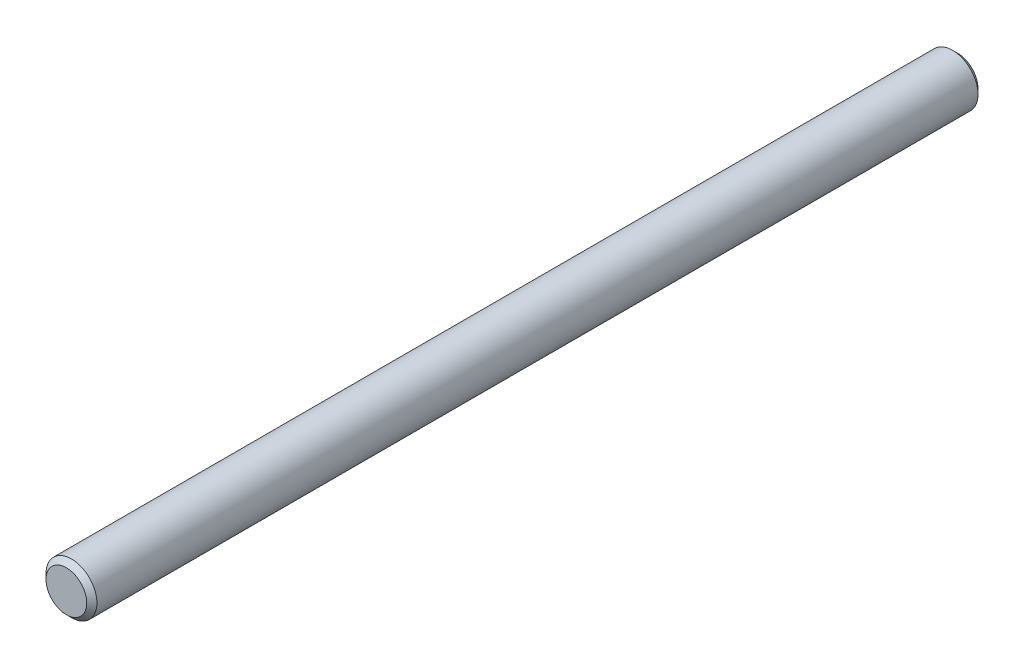
from build123d import *

# Parameters (mm, degrees)
SKETCH1_R           = 1
BOSS_EXTRUDE1_DEPTH = 17.5
CHAMFER1_SIZE       = 0.2


with BuildPart() as part:
    # Sketch1 → Boss-Extrude1 (new, symmetric)
    with BuildSketch(Plane.XY):
        Circle(SKETCH1_R)
    extrude(amount=BOSS_EXTRUDE1_DEPTH, both=True)

    # Chamfer1
    chamfer1_edges = [part.edges().sort_by_distance(p)[0] for p in [
        (-1, 0, -17.5),
        (-1, 0, 17.5),
    ]]
    chamfer(chamfer1_edges, length=CHAMFER1_SIZE)


solid = part.part
